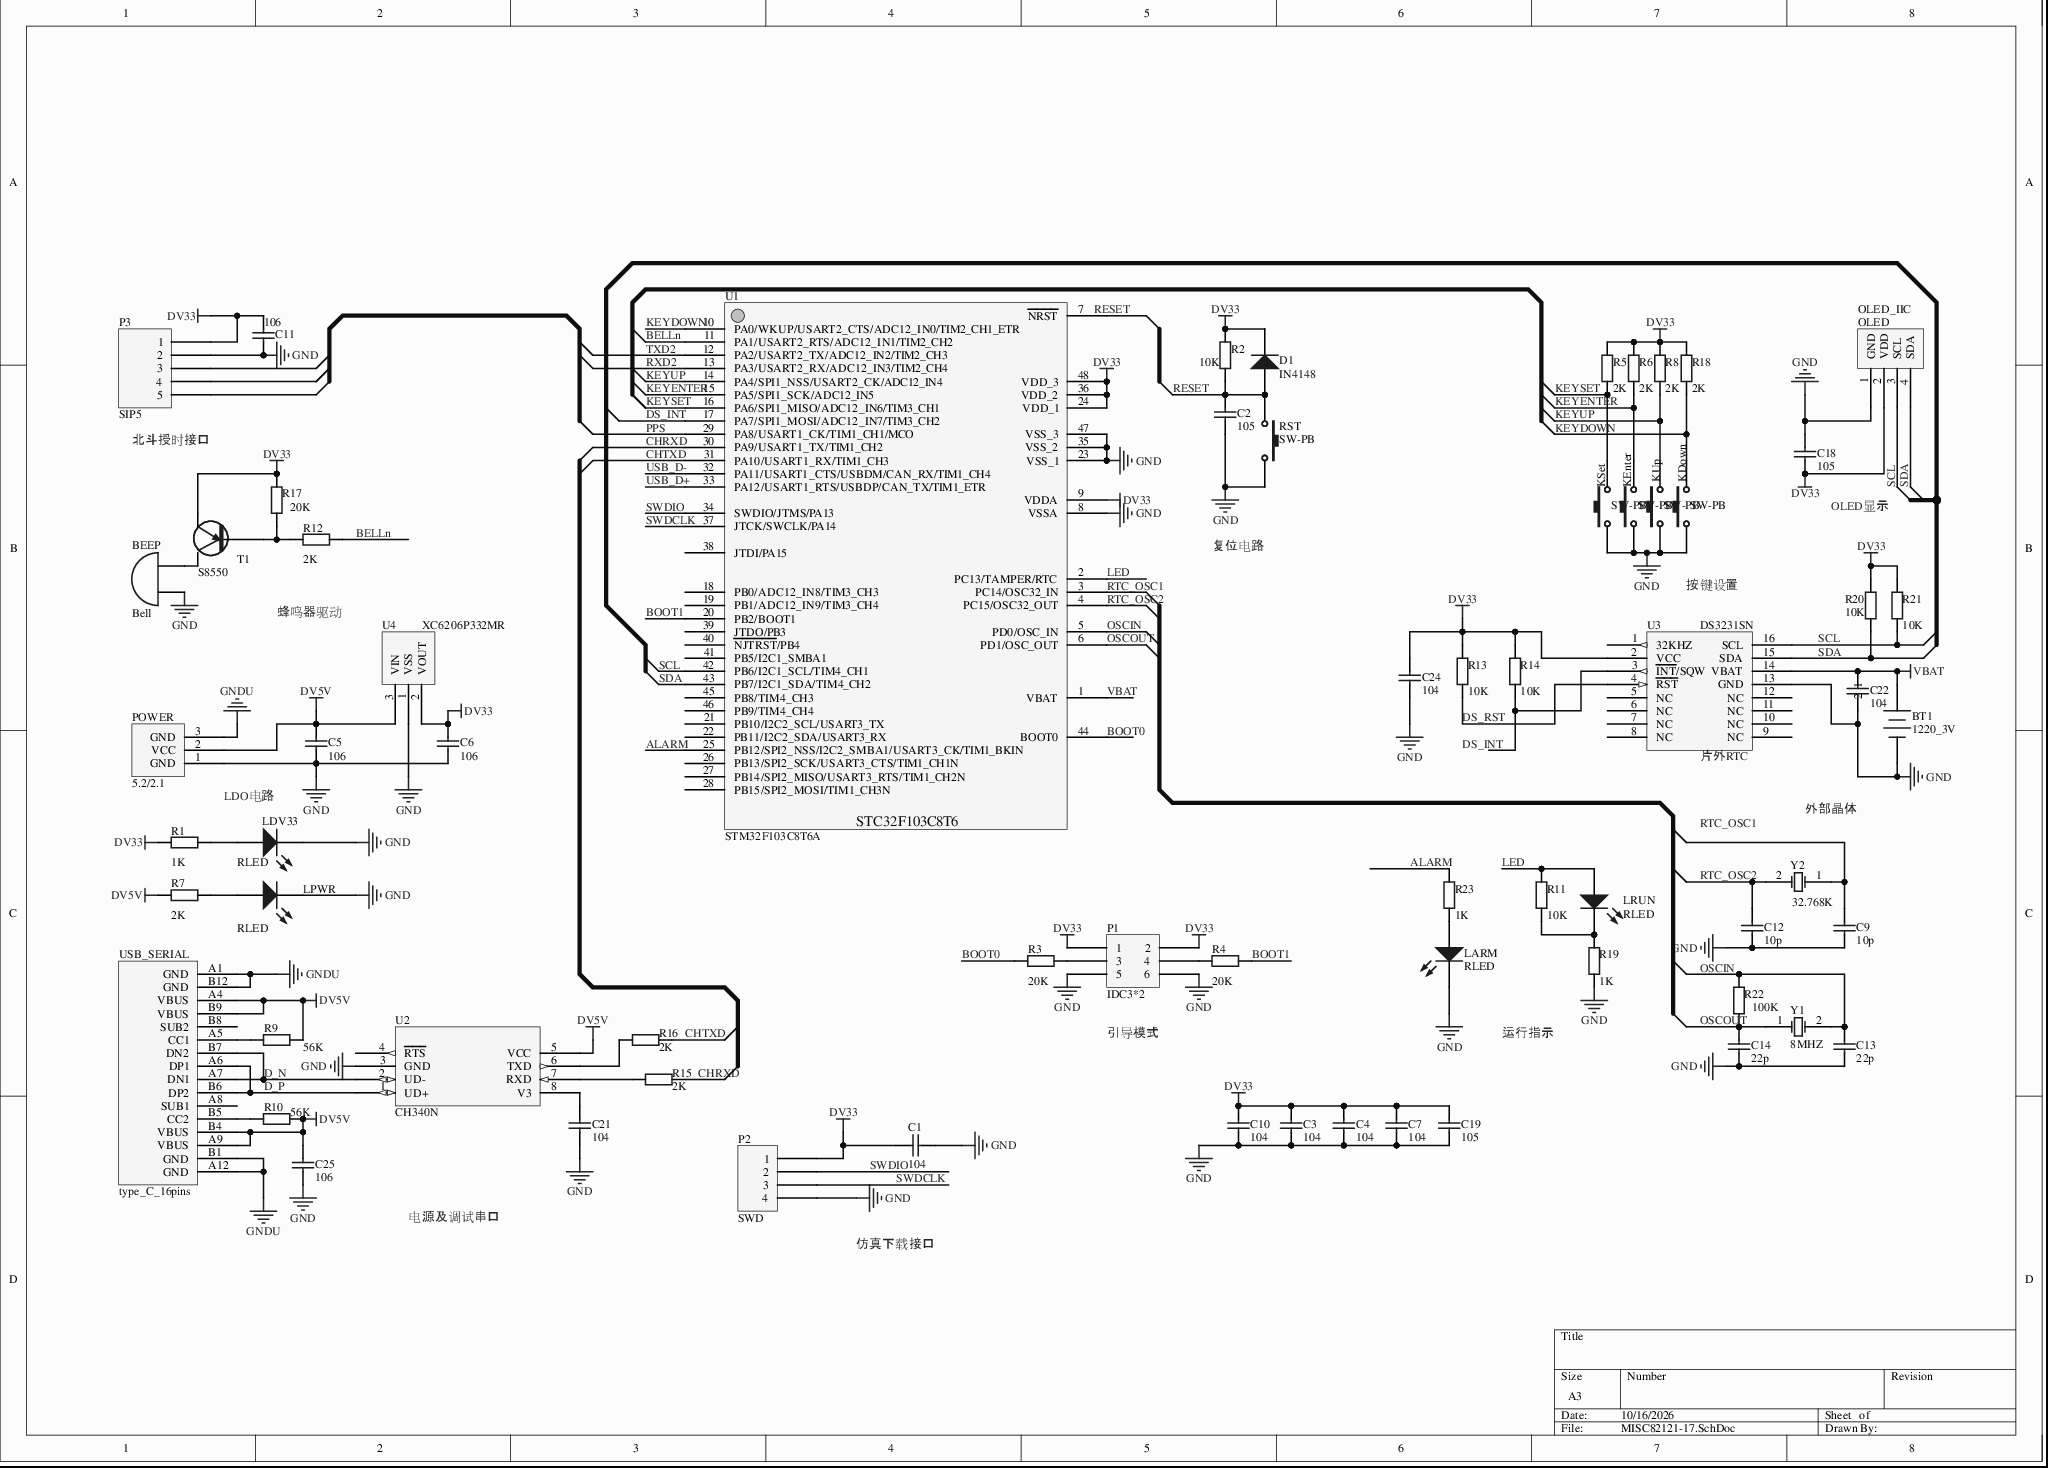
[diagram p0: MISC82121-17.SchDoc]
# Altium project MISC82121-4.PrjPcb
1 sheet, 67 parts. Net scope: global (net labels, ports and power ports of the same name join across sheets).
Board file: MISC82121.PcbDoc

## Sheet MISC82121-17.SchDoc
size A3

### Parts
BEEP  Bell  [HN9650B]
BT1  1220_3V  [CR1220]
C1  104  [C0805]
C2  105  [C0805]
C3  104  [C0805]
C4  104  [C0805]
C5  106  [C0805]
C6  106  [C0805]
C7  104  [C0805]
C9  10p  [C0603]
C10  104  [C0805]
C11  106  [C0805]
C12  10p  [C0603]
C13  22p  [C0603]
C14  22p  [C0603]
C18  105  [C0805]  (net tie, no BOM)
C19  105  [C0805]
C21  104  [C0805]
C22  104  [C0805]  (mechanical)
C24  104  [C0805]
C25  106  [C0805]  (net tie, no BOM)
D1  IN4148  [D0805]
KDown  SW-PB  [KEY_8mm]
KEnter  SW-PB  [KEY_8mm]
KSet  SW-PB  [KEY_8mm]
KUp  SW-PB  [KEY_8mm]
LARM  RLED  [LED0805]
LDV33  RLED  [LED0805]
LPWR  RLED  [LED0805]
LRUN  RLED  [LED0805]
OLED  OLED_IIC  [OLED]
P1  IDC3*2  [HDR2X3]
P2  SWD  [HDR1X4]
P3  SIP5  [HDR1X5]
POWER  5.2/2.1  [SWC_SET]
R1  value 1K  [R0805]  (hidden comment: Res2)
R2  value 10K  [R0805]  (hidden comment: Res2)
R3  value 20K  [R0805]  (hidden comment: Res2)
R4  value 20K  [R0805]  (hidden comment: Res2)
R5  value 2K  [R0805]  (hidden comment: Res2)
R6  value 2K  [R0805]  (hidden comment: Res2)
R7  value 2K  [R0805]  (hidden comment: Res2)
R8  value 2K  [R0805]  (hidden comment: Res2)
R9  value 56K  [R0805]  (hidden comment: Res2)
R10  value 56K  [R0805]  (hidden comment: Res2)
R11  value 10K  [R0805]  (hidden comment: Res2)
R12  value 2K  [R0805]  (hidden comment: Res2)
R13  value 10K  [R0805]  (hidden comment: Res2)
R14  value 10K  [R0805]  (hidden comment: Res2)
R15  value 2K  [R0805]  (hidden comment: Res2)
R16  value 2K  [R0805]  (hidden comment: Res2)
R17  value 20K  [R0805]  (hidden comment: Res2)
R18  value 2K  [R0805]  (hidden comment: Res2)
R19  value 1K  [R0805]  (hidden comment: Res2)
R20  value 10K  [R0805]  (hidden comment: Res2)
R21  value 10K  [R0805]  (hidden comment: Res2)
R22  value 100K  [R0805]  (hidden comment: Res2)
R23  value 1K  [R0805]  (hidden comment: Res2)
RST  SW-PB  [KEY_8mm]
T1  S8550  [SOT-23]
U1  STM32F103C8T6A  [LQFP48]
U2  CH340N  [SO-8]
U3  DS3231SN  [SOP-16]
U4  XC6206P332MR  [SOT-23S]
USB_SERIAL  type_C_16pins  [TYPE_C_16PIN]
Y1  8MHZ  [OSC 5032-2P]
Y2  32.768K  [OSC_2*6]

### Nets
DV5V: C5.2 C25.2 POWER.2(VCC) R7.1 R9.2 R10.2 U2.5(VCC) U4.3(VIN) USB_SERIAL.A4(VBUS) USB_SERIAL.A9(VBUS) USB_SERIAL.B4(VBUS) USB_SERIAL.B9(VBUS)
DV33: C1.1 C3.2 C4.2 C6.2 C7.2 C10.2 C11.2 C18.1 C19.2 C24.2 D1.2(K) OLED.2(VDD) P1.1 P1.2 P2.1 P3.B28(1) R1.1 R2.2 R5.2 R6.2 R8.2 R13.2 R14.2 R17.2 R18.2 R20.2 R21.2 T1.B19 U1.9(VDDA) U1.24(VDD_1) U1.36(VDD_2) U1.48(VDD_3) U3.2(VCC) U4.2(VOUT)
GND: BEEP.1(A) BT1.2(-) C1.2 C2.1 C3.1 C4.1 C5.1 C6.1 C7.1 C9.1 C10.1 C11.1 C12.1 C13.1 C14.1 C18.2 C19.1 C21.2 C22.1 C24.1 C25.1 KDown.1 KEnter.1 KSet.1 KUp.1 LARM.2(K) LDV33.2(K) LPWR.2(K) OLED.1(GND) P1.5 P1.6 P2.4 P3.B27(2) POWER.1(GND) R19.1 RST.2 U1.8(VSSA) U1.23(VSS_1) U1.35(VSS_2) U1.47(VSS_3) U2.3(GND) U3.13(GND) U4.1(VSS)
GNDU: POWER.3(GND) USB_SERIAL.A1(GND) USB_SERIAL.A12(GND) USB_SERIAL.B1(GND) USB_SERIAL.B12(GND)
VBAT: BT1.1(+) C22.2 U1.1(VBAT) U3.14(VBAT)
ALARM: R23.2 U1.25(PB12/SPI2_NSS/I2C2_SMBA1/USART3_CK/TIM1_BKIN)
BELLn: R12.2 U1.11(PA1/USART2_RTS/ADC12_IN1/TIM2_CH2)
BOOT0: R3.1 U1.44(BOOT0)
BOOT1: R4.2 U1.20(PB2/BOOT1)
CHRXD: R15.2 U1.30(PA9/USART1_TX/TIM1_CH2)
CHTXD: R16.2 U1.31(PA10/USART1_RX/TIM1_CH3)
D_N: U2.2(UD-) USB_SERIAL.A7(DN1) USB_SERIAL.B7(DN2)
D_P: U2.1(UD+) USB_SERIAL.A6(DP1) USB_SERIAL.B6(DP2)
DS_INT: U1.17(PA7/SPI1_MOSI/ADC12_IN7/TIM3_CH2)
DS_RST: R13.1 U3.4(~{RST})
KEYDOWN: KDown.2 R18.1 U1.10(PA0/WKUP/USART2_CTS/ADC12_IN0/TIM2_CH1_ETR)
KEYENTER: KEnter.2 R6.1 U1.15(PA5/SPI1_SCK/ADC12_IN5)
KEYSET: KSet.2 R5.1 U1.16(PA6/SPI1_MISO/ADC12_IN6/TIM3_CH1)
KEYUP: KUp.2 R8.1 U1.14(PA4/SPI1_NSS/USART2_CK/ADC12_IN4)
LED: LRUN.1(A) R11.2 U1.2(PC13/TAMPER/RTC)
OSCIN: C13.2 R22.2 U1.5(PD0/OSC_IN) Y1.2(OSC2)
OSCOUT: C14.2 R22.1 U1.6(PD1/OSC_OUT) Y1.1(OSC1)
PPS: U1.29(PA8/USART1_CK/TIM1_CH1/MCO)
RESET: C2.2 D1.1(A) R2.1 RST.1
RTC_OSC1: U1.3(PC14/OSC32_IN)
RTC_OSC2: C12.2 U1.4(PC15/OSC32_OUT) Y2.2(OSC2)
RXD2: U1.13(PA3/USART2_RX/ADC12_IN3/TIM2_CH4)
SCL: OLED.3(SCL) R21.1 U1.42(PB6/I2C1_SCL/TIM4_CH1) U3.16(SCL)
SDA: OLED.4(SDA) R20.1 U1.43(PB7/I2C1_SDA/TIM4_CH2) U3.15(SDA)
SWDCLK: P2.3 U1.37(JTCK/SWCLK/PA14)
SWDIO: P2.2 U1.34(SWDIO/JTMS/PA13)
TXD2: U1.12(PA2/USART2_TX/ADC12_IN2/TIM2_CH3)
USB_D+: U1.33(PA12/USART1_RTS/USBDP/CAN_TX/TIM1_ETR)
USB_D-: U1.32(PA11/USART1_CTS/USBDM/CAN_RX/TIM1_CH4)
NetBEEP_2: BEEP.2(B) T1.B20
NetC9_2: C9.2 Y2.1(OSC1)
NetC21_1: C21.1 U2.8(V3)
NetLARM_1: LARM.1(A) R23.1
NetLDV33_1: LDV33.1(A) R1.2
NetLPWR_1: LPWR.1(A) R7.2
NetLRUN_2: LRUN.2(K) R11.1 R19.2
NetP1_3: P1.3 R3.2
NetP1_4: P1.4 R4.1
NetR9_1: R9.1 USB_SERIAL.A5(CC1)
NetR10_1: R10.1 USB_SERIAL.B5(CC2)
NetR12_1: R12.1 R17.1 T1.B21
NetR14_1: R14.1 U3.3(~{INT}/SQW)
NetR15_1: R15.1 U2.7(RXD)
NetR16_1: R16.1 U2.6(TXD)

Not connected (* = marked no-connect by the designer): P3 B24(5)* B25(4)* B26(3)*; U1 7(~{NRST}) 18(PB0/ADC12_IN8/TIM3_CH3) 19(PB1/ADC12_IN9/TIM3_CH4) 21(PB10/I2C2_SCL/USART3_TX) 22(PB11/I2C2_SDA/USART3_RX) 26(PB13/SPI2_SCK/USART3_CTS/TIM1_CH1N) 27(PB14/SPI2_MISO/USART3_RTS/TIM1_CH2N) 28(PB15/SPI2_MOSI/TIM1_CH3N) 38(JTDI/PA15) 39(JTDO/PB3) 40(~{NJTRST}/PB4) 41(PB5/I2C1_SMBA1) 45(PB8/TIM4_CH3) 46(PB9/TIM4_CH4); U2 4(~{RTS}); U3 1(32KHZ)* 5(NC) 6(NC) 7(NC) 8(NC) 9(NC) 10(NC) 11(NC) 12(NC); USB_SERIAL A8(SUB1) B8(SUB2)

### Layout directives
differential pair: D_N, D_P

### Notes on the sheet
- Labels drawn without touching a wire or pin: DS_INT, LDO电路, OLED显示, PERSON_A, RESET, RTC_OSC1, 仿真下载接口, 北斗授时接口, 复位电路, 外部晶体, 引导模式, 按键设置, 片外RTC, 电源及调试串口, 蜂鸣器驱动, 运行指示

### Library data of the parts
BEEP = Bell: Electrical Bell; Published: 24-Mar-1999; LatestRevisionDate: 17-Jul-2002; LatestRevisionNote: Re-released for DXP Platform.; PackageReference: PIN2; Publisher: Altium Limited
BT1 = Battery: Multicell Battery; Published: 24-Mar-1999; LatestRevisionDate: 17-Jul-2002; LatestRevisionNote: Re-released for DXP Platform.; PackageReference: BAT-2; PackageDescription: Battery; 2 Leads; Publisher: Altium Limited
C1-C7 C9-C14 C18 C19 C21 C22 C24 C25 = Cap: Capacitor; Published: 8-Jun-2000; LatestRevisionDate: 17-Jul-2002; LatestRevisionNote: Re-released for DXP Platform.; PackageReference: RAD-0.3; PackageDescription: Radial Cap, Thru-Hole; 2 Leads; 0.3 in Pin Spacing; Publisher: Altium Limited
  C1 C3 C4 C7 C10 C21 C22 C24: Value: 104
  C2 C18 C19: Value: 105
  C5 C6 C11 C25: Value: 106
  C9 C12: Value: 10p
  C13 C14: Value: 22p
D1 = Diode: Default Diode; Published: 8-Jun-2000; LatestRevisionDate: 17-Jul-2002; LatestRevisionNote: Re-released for DXP Platform.; PackageVersion: Sep-1996; PackageReference: SMC; PackageDescription: DO-214-AB/SMC; 2 C-Bend Leads; Body 7.9 x 5.9 mm, inc. leads (LxW); Code_JEDEC: DO-214-AB; Publisher: Altium Limited
KDown KEnter KSet KUp RST = SW-PB: Switch; Published: 24-Mar-1999; LatestRevisionDate: 17-Jul-2002; LatestRevisionNote: Re-released for DXP Platform.; PackageReference: SPST-2; PackageDescription: Switch; 2 Leads; Publisher: Altium Limited
LARM LDV33 LPWR LRUN = LED0: Typical INFRARED GaAs LED; Published: 8-Jun-2000; LatestRevisionDate: 08-Jul-2005; LatestRevisionNote: Mech Layer 1 removed.; PackageReference: LED-0; PackageDescription: LED; 2 Leads; Publisher: Altium Limited
OLED = OLED_I2C_I2164
R1-R23 = Res2: Resistor; Published: 8-Jun-2000; LatestRevisionDate: 17-Jul-2002; LatestRevisionNote: Re-released for DXP Platform.; PackageReference: AXIAL-0.4; PackageDescription: Axial Device, Thru-Hole; 2 Leads; 0.4 in Pin Spacing; Publisher: Altium Limited
U1 = STM32F103C8T6
Y1 Y2 = XTAL: Crystal Oscillator; Published: 8-Jun-2000; LatestRevisionDate: 17-Jul-2002; LatestRevisionNote: Re-released for DXP Platform.; PackageReference: R38; PackageDescription: Crystal, Thru-Hole; 2 Leads; Body 3.1 x 8.2 mm (Dia.xH); Publisher: Altium Limited